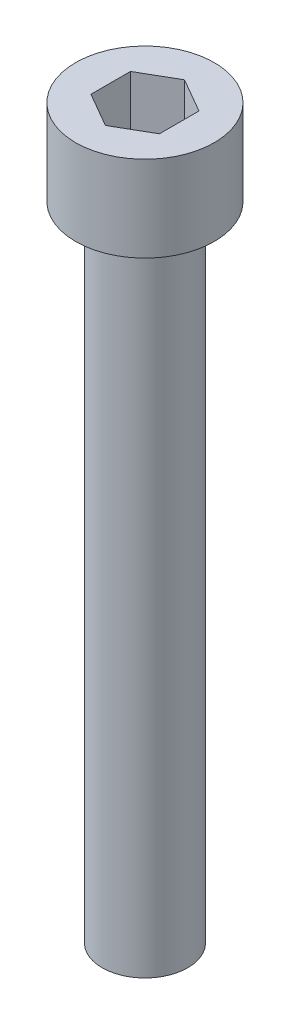
SolidWorks part; units mm, degrees
ref_plane "Front Plane" through (0, 0, 0) normal (0, 0, 1) x (1, 0, 0)
ref_plane "Top Plane" through (0, 0, 0) normal (0, 1, 0) x (1, 0, 0)
ref_plane "Right Plane" through (0, 0, 0) normal (1, 0, 0) x (0, 0, -1)
sketch "Sketch 1" plane through (0, 0, 0) normal (0, 0, 1) x (1, 0, 0)
  line L0 (0, 11.322) -> (0, -25.8305) construction
  line L1 (-9.8983, 0) -> (13.1525, 0) construction
  line L2 (0, 10) -> (-8.1, 10)
  line L3 (-8.1, 10) -> (-8.1, 0)
  line L4 (-8.1, 0) -> (-5, 0)
  line L5 (-5, 0) -> (-5, -75)
  line L6 (-5, -75) -> (0, -75)
  line L7 (0, -75) -> (0, 10)
  dimension "D1" = 10
  dimension "D2" = 75
  dimension "D3" = 10
  dimension "D4" = 16.2
revolve "Revolve 1" add sketch "Sketch 1" angle 360 about L0
sketch "Sketch 2" plane through (0, 10, 0) normal (0, 1, 0) x (1, 0, 0)
  line L1 (0, 4.6188) -> (-4, 2.3094)
  line L2 (-4, 2.3094) -> (-4, -2.3094)
  line L3 (-4, -2.3094) -> (0, -4.6188)
  line L4 (0, -4.6188) -> (4, -2.3094)
  line L5 (4, -2.3094) -> (4, 2.3094)
  line L6 (4, 2.3094) -> (0, 4.6188)
  circle A0 centre (0, 0) radius 4 construction
  dimension "D1" = 8
extrude "Cut-Extrude 1" cut sketch "Sketch 2" against normal blind 6
